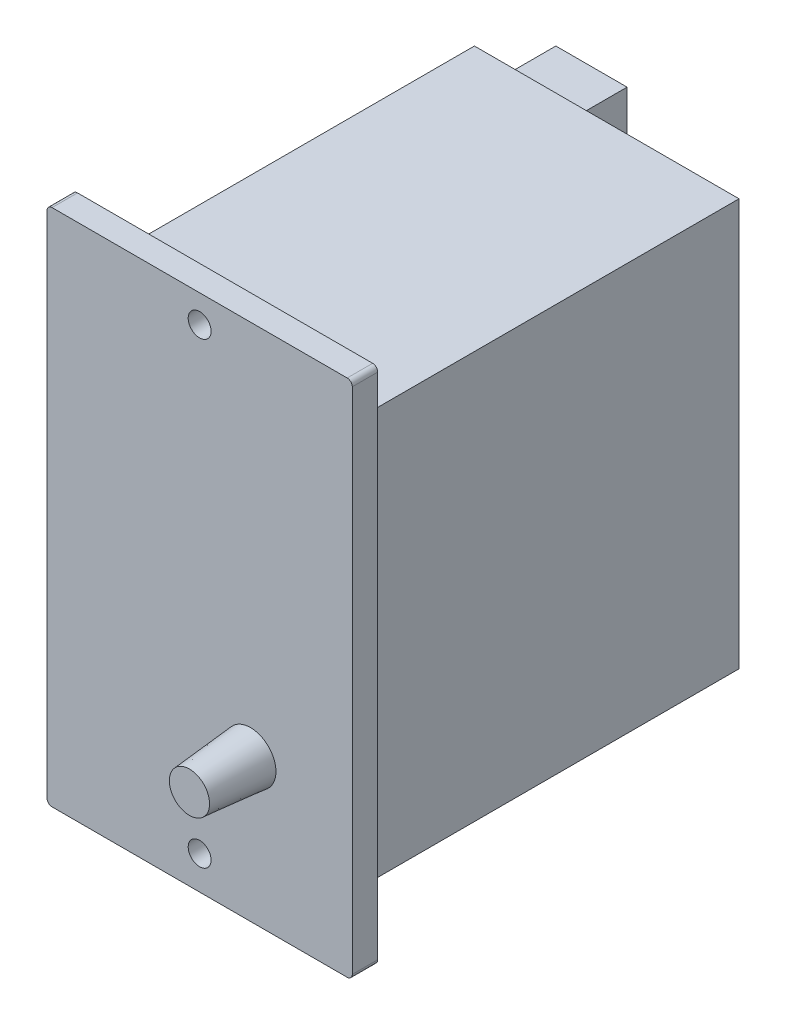
SolidWorks part; units mm, degrees
ref_plane "前视基准面" through (0, 0, 0) normal (0, 0, 1) x (1, 0, 0)
ref_plane "上视基准面" through (0, 0, 0) normal (0, 1, 0) x (1, 0, 0)
ref_plane "右视基准面" through (0, 0, 0) normal (1, 0, 0) x (0, 0, -1)
sketch "草图1" plane through (0, 0, 0) normal (0, 0, 1) x (1, 0, 0)
  line L1 (-30, -51) -> (30, -51)
  line L2 (-30, -51) -> (-30, 51)
  line L3 (-30, 51) -> (30, 51)
  line L4 (30, -51) -> (30, 51)
  line L5 (-30, -51) -> (30, 51) construction
  line L6 (-30, 51) -> (30, -51) construction
  circle A0 centre (0, 45.5635) radius 2.25
  circle A1 centre (0, -44.4365) radius 2.25
  point P0 (0, 0)
  dimension "D3" = 90
  dimension "D4" = 4.5
  dimension "D5" = 30
  dimension "D1" = 60
  dimension "D2" = 102
extrude "凸台-拉伸1" add sketch "草图1" along normal blind 5
sketch "草图2" plane through (0, 0, 0) normal (0, 0, -1) x (-1, 0, 0)
  line L1 (-26, -40) -> (26, -40)
  line L2 (-26, -40) -> (-26, 40)
  line L3 (-26, 40) -> (26, 40)
  line L4 (26, -40) -> (26, 40)
  line L5 (-26, -40) -> (26, 40) construction
  line L6 (-26, 40) -> (26, -40) construction
  point P0 (0, 0)
  dimension "D1" = 52
  dimension "D2" = 80
extrude "凸台-拉伸2" add sketch "草图2" along normal blind 75
sketch "草图3" plane through (0, 0, 5) normal (0, 0, 1) x (1, 0, 0)
  line L0 (-30, 51) -> (-30, -51) construction
  line L1 (-30, -51) -> (30, -51) construction
  circle A0 centre (10, -23) radius 5
  dimension "D1" = 10
  dimension "D2" = 40
  dimension "D3" = 28
extrude "凸台-拉伸3" add sketch "草图3" along normal blind 12 draft 5
fillet "圆角1" radius 1 4 edges at (-30, -51, 2.5) (30, -51, 2.5) (30, 51, 2.5) (-30, 51, 2.5)
sketch "草图4" plane through (0, 0, -75) normal (0, 0, -1) x (-1, 0, 0)
  line L0 (26, -40) -> (26, 40) construction
  line L1 (8, 36) -> (22, 36)
  line L2 (8, 36) -> (8, -36)
  line L3 (8, -36) -> (22, -36)
  line L4 (22, 36) -> (22, -36)
  line L5 (26, 40) -> (-26, 40) construction
  dimension "D1" = 72
  dimension "D2" = 14
  dimension "D3" = 4
  dimension "D4" = 4
extrude "凸台-拉伸4" add sketch "草图4" along normal blind 12
